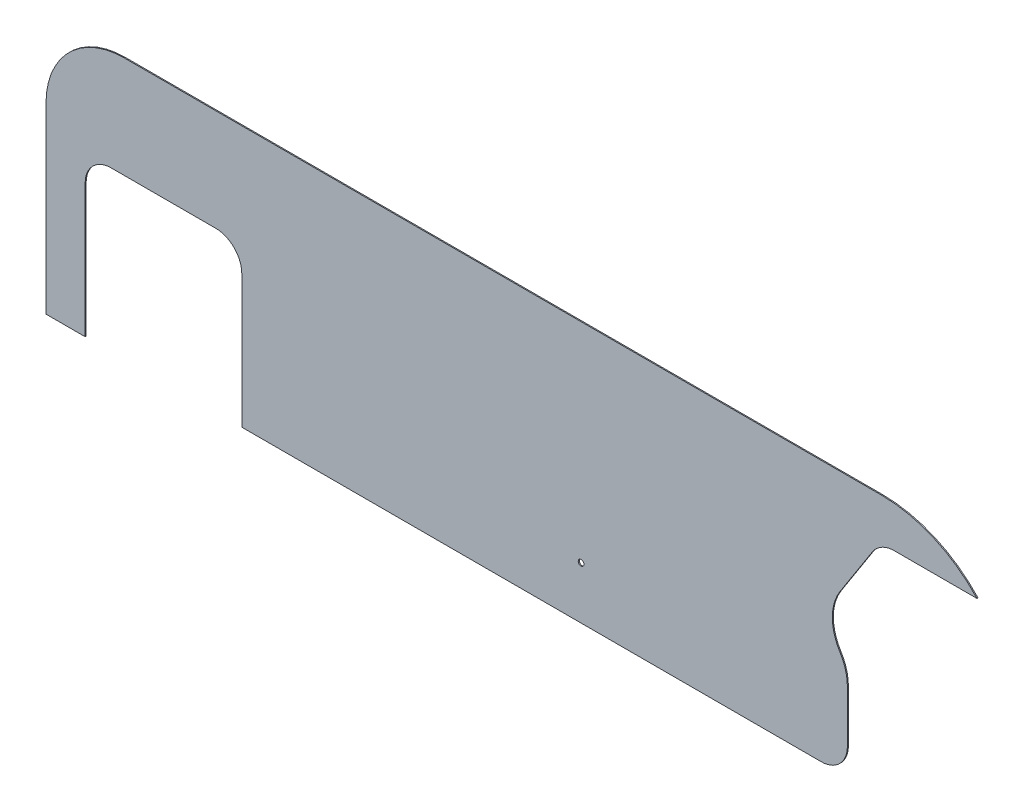
from build123d import *

# Parameters (mm, degrees)
SKETCH1_R           = 5.588
BOSS_EXTRUDE1_DEPTH = 1


with BuildPart() as part:
    # Sketch1 → Boss-Extrude1 (new, symmetric)
    with BuildSketch(Plane.XY):
        with BuildLine():
            Line((186.235876243, 172.72), (25.4, 172.72))
            ThreePointArc((25.4, 172.72), (1.035545712, 166.495928114), (-17.35858909, 149.348872727))
            Line((-17.35858909, 149.348872727), (-80.172354543, 51.429136363))
            ThreePointArc((-80.172354543, 51.429136363), (-95.248979697, 0.440870364), (-80.645, -50.684775574))
            ThreePointArc((-80.645, -50.684775574), (-69.764050811, -74.996020383), (-66.04, -101.369551148))
            Line((-66.04, -101.369551148), (-66.04, -203.2))
            ThreePointArc((-66.04, -203.2), (-80.918975516, -239.121024484), (-116.84, -254))
            Line((-116.84, -254), (-1244.6, -254))
            Line((-1244.6, -254), (-1244.6, 5.08))
            ThreePointArc((-1244.6, 5.08), (-1259.478975516, 41.001024484), (-1295.4, 55.88))
            Line((-1295.4, 55.88), (-1498.6, 55.88))
            ThreePointArc((-1498.6, 55.88), (-1534.521024484, 41.001024484), (-1549.4, 5.08))
            Line((-1549.4, 5.08), (-1549.4, -254))
            Line((-1549.4, -254), (-1625.6, -254))
            Line((-1625.6, -254), (-1625.6, 101.6))
            ThreePointArc((-1625.6, 101.6), (-1580.963073453, 209.363073453), (-1473.2, 254))
            Line((-1473.2, 254), (0, 254))
            ThreePointArc((0, 254), (101.6, 232.794845304), (186.235876243, 172.72))
        make_face()
        with Locations((-584.2, -152.4)):
            Circle(SKETCH1_R, mode=Mode.SUBTRACT)
    extrude(amount=BOSS_EXTRUDE1_DEPTH, both=True)


solid = part.part
